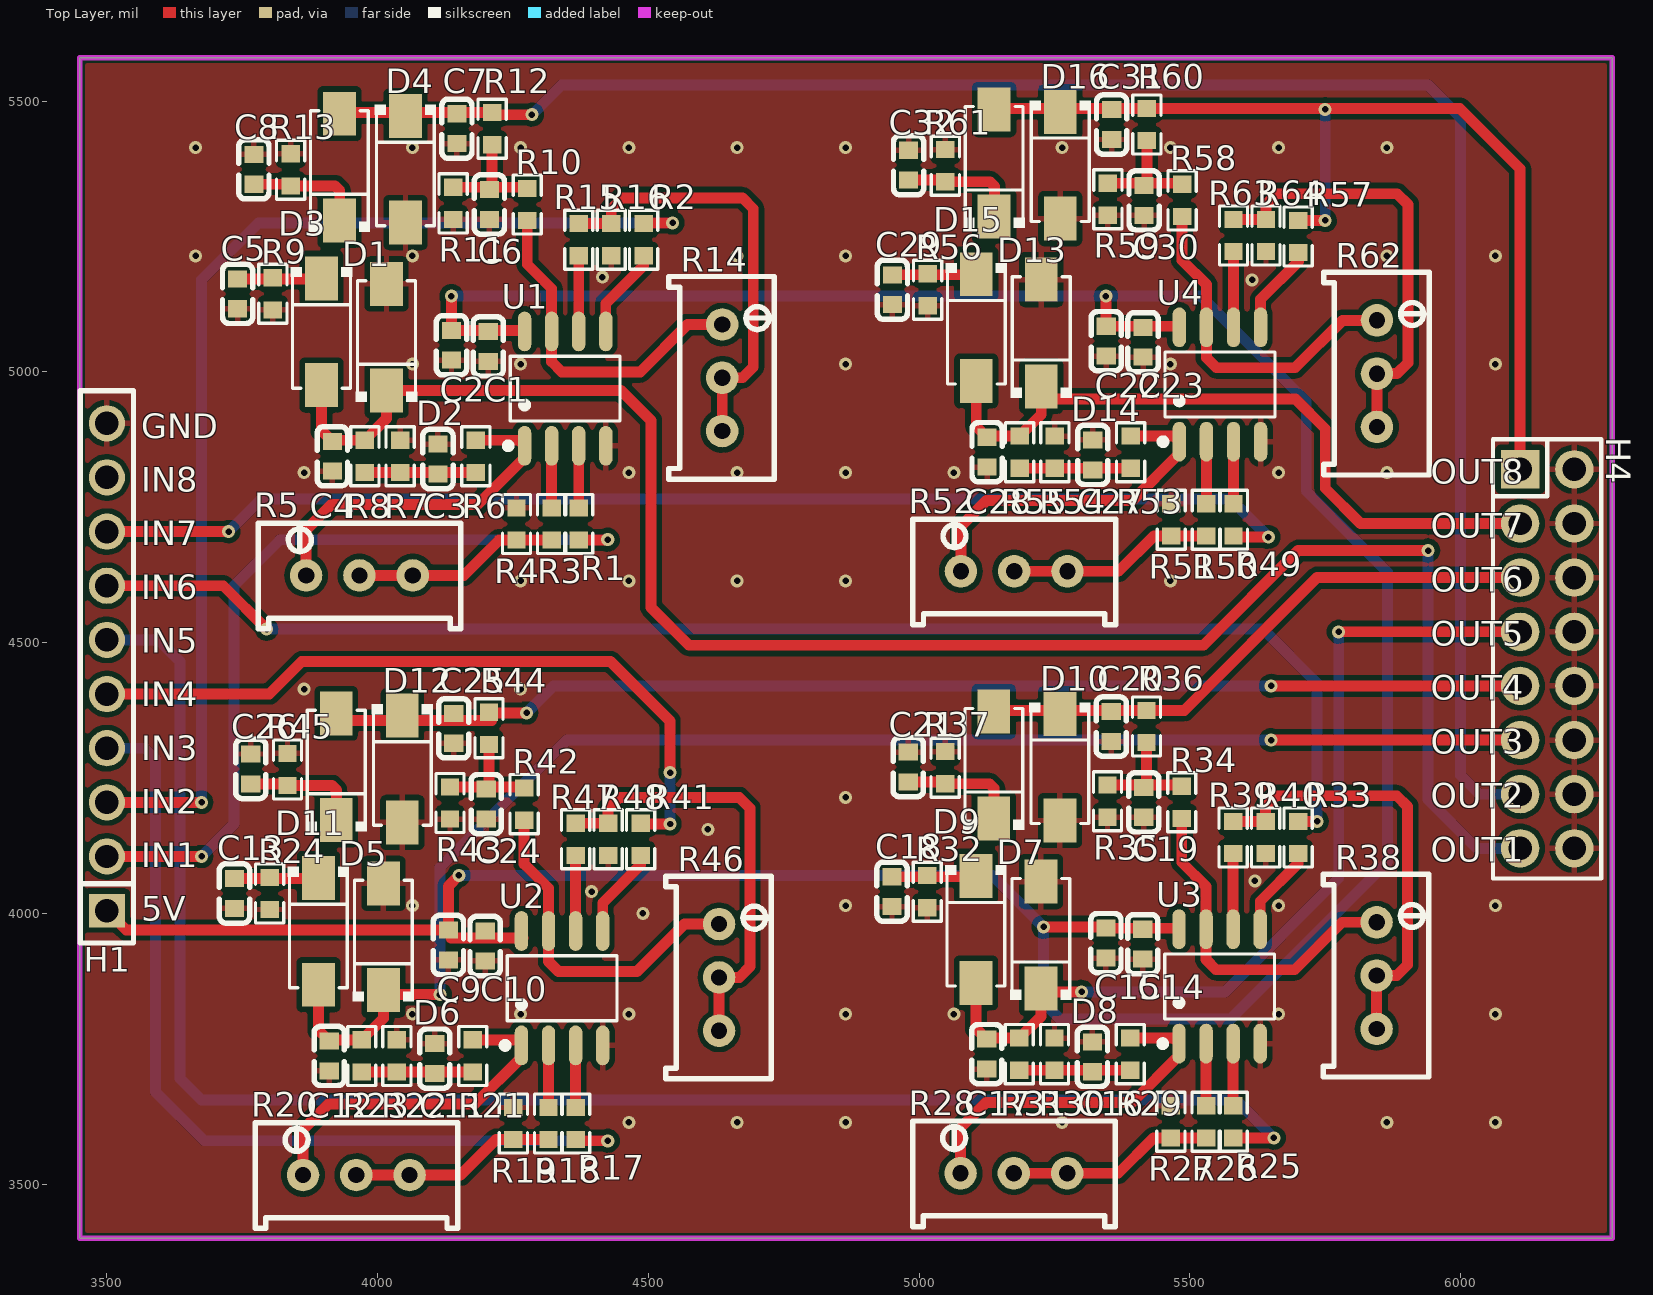
[diagram p0: Top Layer view]
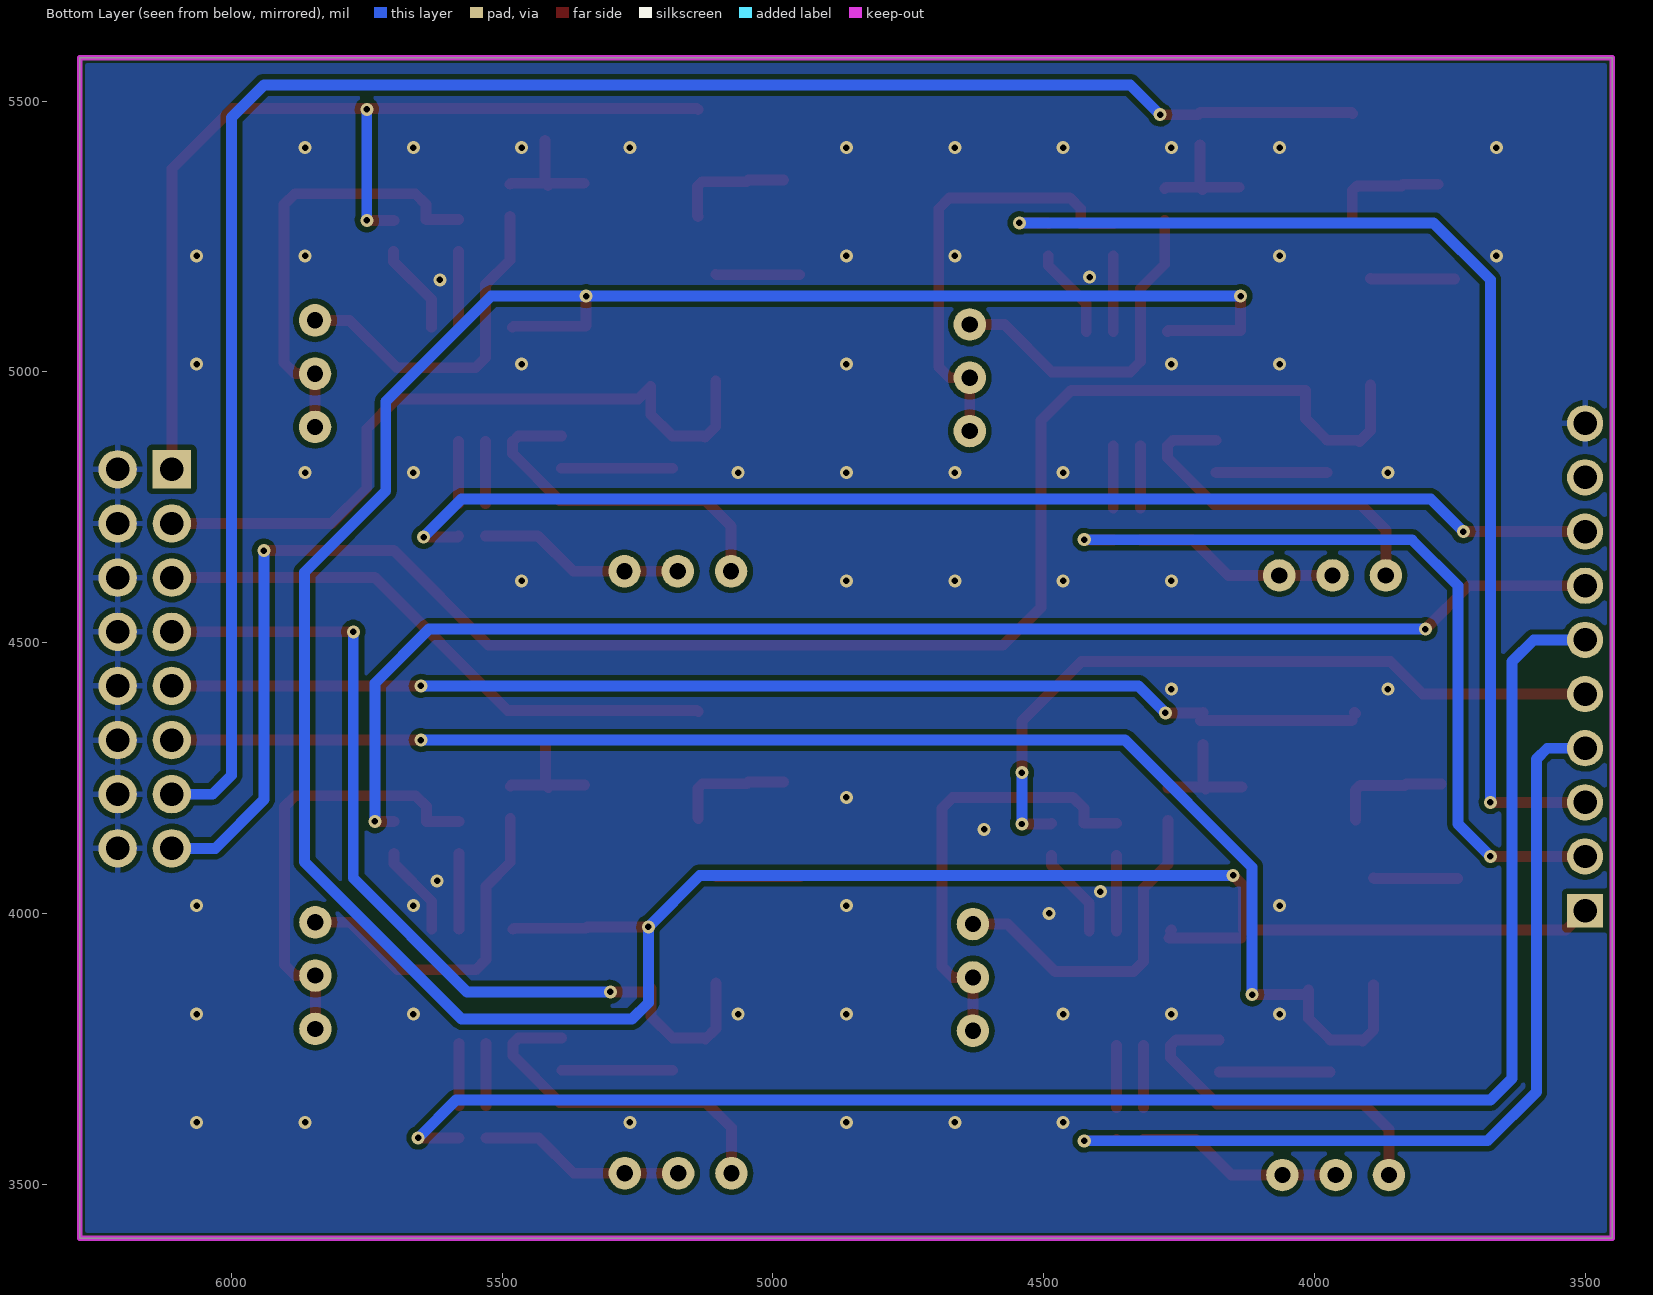
[diagram p1: Bottom Layer view, seen from below]
# Altium PCB MISC49941.pcbdoc
Units mil, origin at the board's own origin, x right, y up, seen from the top; angles counter-clockwise.
Board outline 2830 x 2180 mil, 2 copper layers (Top Layer, Bottom Layer), stack 62.206 mil thick; 118 components, 66 nets, 290 pads, 85 vias.

## Layer stack, top to bottom
Top Solder Mask Layer: solder mask 0.394, Dk 3.3
Top Layer: signal copper 1.379
Dielectric1: surface 59.449, FR4, Dk 4.5
Bottom Layer: signal copper 1.378
Bottom Solder Mask Layer: solder mask 0.394, Dk 3.3

## Board outline
3450,5580 3450,3400 6280,3400 6280,5580

## Design rules (kind name [scope] priority, off if disabled: settings)
BoardOutlineClearance copperThickness2oz_1 [All] p2 off: genericclearance=7.99 ignorepadtopadclearanceinfootprint=FALSE except(0: Arc-SplitContinuation Track-SplitContinuation SMDPad-SplitContinuation THPad-SplitContinuation Via-SplitContinuation Fill-SplitContinuation Region-SplitContinuation Poly-SplitContinuation Text-SplitContinuation Hole-SplitContinuation; 5.98: Arc-CutoutEdge SMDPad-CutoutEdge THPad-CutoutEdge Via-CutoutEdge Fill-CutoutEdge Region-CutoutEdge Text-CutoutEdge; 6.93: Hole-OutlineEdge Hole-CutoutEdge; 10: Poly-OutlineEdge Poly-CutoutEdge; 11.81: Arc-OutlineEdge Track-OutlineEdge SMDPad-OutlineEdge THPad-OutlineEdge Via-OutlineEdge Fill-OutlineEdge Region-OutlineEdge Text-OutlineEdge Track-CutoutEdge)
BoardOutlineClearance copperThickness1oz_1 [All] p4: genericclearance=4.02 ignorepadtopadclearanceinfootprint=FALSE except(0: Arc-SplitContinuation Track-SplitContinuation SMDPad-SplitContinuation THPad-SplitContinuation Via-SplitContinuation Fill-SplitContinuation Region-SplitContinuation Poly-SplitContinuation Text-SplitContinuation Hole-SplitContinuation; 6: SMDPad-CutoutEdge THPad-CutoutEdge Via-CutoutEdge Fill-CutoutEdge Region-CutoutEdge Text-CutoutEdge; 6.93: Hole-OutlineEdge Hole-CutoutEdge; 10: Poly-OutlineEdge Poly-CutoutEdge; 11.8: Arc-OutlineEdge Track-OutlineEdge SMDPad-OutlineEdge THPad-OutlineEdge Via-OutlineEdge Fill-OutlineEdge Region-OutlineEdge Text-OutlineEdge; 11.81: Arc-CutoutEdge Track-CutoutEdge)
Clearance copperThickness2oz [All] p1 off: gap=7.99 ignorepadtopadclearanceinfootprint=FALSE except(5.98: SMDPad-Track SMDPad-SMDPad THPad-Track SMDPad-THPad THPad-THPad Track-Via SMDPad-Via THPad-Via Via-Via Fill-Track Region-Track Fill-SMDPad Region-SMDPad Fill-THPad Region-THPad Fill-Via Region-Via Fill-Fill Fill-Region Region-Region Arc-Track Arc-SMDPad Arc-THPad Arc-Via Fill-Arc Region-Arc Arc-Arc Text-Track SMDPad-Text Text-THPad Text-Via Fill-Text Region-Text Arc-Text Text-Text; 6.93: Hole-Track Hole-SMDPad Hole-THPad Hole-Via Fill-Hole Region-Hole Hole-Arc Hole-Text; 10: Poly-Track Poly-SMDPad Poly-THPad Poly-Via Poly-Fill Poly-Region Poly-Poly Poly-Arc Poly-Text Poly-Hole)
Clearance copperThickness1oz [All] p3: gap=4.02 ignorepadtopadclearanceinfootprint=FALSE except(5.98: SMDPad-Track SMDPad-SMDPad THPad-Track SMDPad-THPad THPad-THPad Track-Via SMDPad-Via THPad-Via Via-Via Fill-Track Region-Track Fill-SMDPad Region-SMDPad Fill-THPad Region-THPad Fill-Via Region-Via Fill-Fill Fill-Region Region-Region; 6: Arc-Track Arc-SMDPad Arc-THPad Arc-Via Fill-Arc Region-Arc Arc-Arc Text-Track SMDPad-Text Text-THPad Text-Via Fill-Text Region-Text Arc-Text Text-Text; 6.93: Hole-Track Hole-SMDPad Hole-THPad Hole-Via Fill-Hole Region-Hole Hole-Arc Hole-Text; 10: Poly-Track Poly-SMDPad Poly-THPad Poly-Via Poly-Fill Poly-Region Poly-Poly Poly-Arc Poly-Text Poly-Hole)
Creepage creepage [All] p1: checkdistance=0 ignoreinternallayers=TRUE applytopolygonpour=TRUE
DiffPairsRouting differentialPair [All] p1: maxlimit=6 minlimit=6 mostfreqgap=6 toplayer_minwidth=5 toplayer_prefwidth=10 toplayer_maxwidth=100 toplayer_mingap=6 toplayer_prefgap=6 toplayer_maxgap=6 bottomlayer_minwidth=5 bottomlayer_prefwidth=10 bottomlayer_maxwidth=100 bottomlayer_mingap=6 bottomlayer_prefgap=6 bottomlayer_maxgap=6 maxuncoupledlength=10
HoleToHoleClearance otherClearance [All] p1: gap=11.81 allowstackedmicrovias=TRUE
Length netLength [All] p1: minlimit=0 maxlimit=0
MatchedLengths netLengthTolerance [All] p1: tolerance=1000
PasteMaskExpansion pasteMaskExpansion [All] p1: expansion=0
PlaneConnect innerPlane [All] p1: planeconnectstyle=Relief reliefexpansion=20 reliefentries=4 reliefconductorwidth=10 reliefairgap=10
PolygonConnect copperRegion [(InNet('GND'))] p1: connectstyle=Relief reliefconductorwidth=10 reliefentries=4 polygonreliefangle="90 Angle" airgapwidth=10 via.connectstyle=Relief via.reliefconductorwidth=10 via.reliefentries=4 via.polygonreliefangle="90 Angle" via.airgapwidth=10
RoutingVias viaSize [All] p1: holewidth=12.01 width=24.02 viastyle="Through Hole" minholewidth=11.81 minwidth=19.68 maxholewidth=248.03 maxwidth=393.7
SolderMaskExpansion solderMaskExpansion [IsVia] p1: expansion=-1000 istentingtop=TRUE
SolderMaskExpansion solderMaskExpansion [All] p2: expansion=2 istentingtop=FALSE
Width copperThickness2oz_2 [All] p1 off: maxlimit=100 minlimit=8 preferedwidth=10
Width copperThickness1oz_2 [All] p2: maxlimit=100 minlimit=5 preferedwidth=10

## Components (designator, comment, footprint, x,y, rotation, side; value= is the part's Value field where it differs from the comment)
C1 "100nF" C0603 4204.38,5047.12 r90 top
C2 "10uF" C0603 4136.4,5049.1 r90 top
C3 "10uF" C0603 4111.4,4839.1 r270 top
C4 "100nF" C0603 3916.4,4844.1 r90 top
C5 "100nF" C0603 3741.4,5144.1 r90 top
C6 "10uF" C0603 4206.4,5309.1 r90 top
C7 "100nF" C0603 4146.4,5449.1 r90 top
C8 "100nF" C0603 3771.4,5374.1 r270 top
C9 "100nF" C0603 4130.63,3941.71 r90 top
C10 "10uF" C0603 4198.61,3939.74 r90 top
C11 "10uF" C0603 4105.63,3731.71 r270 top
C12 "100nF" C0603 3910.63,3736.71 r90 top
C13 "100nF" C0603 3735.63,4036.71 r90 top
C14 "100nF" C0603 5412.98,3943.02 r90 top
C15 "10uF" C0603 5344.99,3945 r90 top
C16 "10uF" C0603 5319.99,3735 r270 top
C17 "100nF" C0603 5124.99,3740 r90 top
C18 "100nF" C0603 4949.99,4040 r90 top
C19 "10uF" C0603 5414.99,4205 r90 top
C20 "100nF" C0603 5354.99,4345 r90 top
C21 "100nF" C0603 4979.99,4270 r270 top
C22 "100nF" C0603 5345.63,5056.71 r90 top
C23 "10uF" C0603 5413.61,5054.74 r90 top
C24 "10uF" C0603 4200.63,4201.71 r90 top
C25 "100nF" C0603 4140.63,4341.71 r90 top
C26 "100nF" C0603 3765.63,4266.71 r270 top
C27 "10uF" C0603 5320.63,4846.71 r270 top
C28 "100nF" C0603 5125.63,4851.71 r90 top
C29 "100nF" C0603 4950.63,5151.71 r90 top
C30 "10uF" C0603 5415.63,5316.71 r90 top
C31 "100nF" C0603 5355.63,5456.71 r90 top
C32 "100nF" C0603 4980.63,5381.71 r270 top
D1 "SS54" SMA_L4.4-W2.8-LS5.4-R-RD 3896.4,5074.1 r270 top
D2 "SS54" SMA_L4.4-W2.8-LS5.4-R-RD 4016.4,5064.1 r90 top
D3 "SS54" SMA_L4.4-W2.8-LS5.4-R-RD 3929.38,5378.12 r90 top
D4 "SS54" SMA_L4.4-W2.8-LS5.4-R-RD 4051.4,5374.1 r270 top
D5 "SS54" SMA_L4.4-W2.8-LS5.4-R-RD 3890.63,3966.71 r270 top
D6 "SS54" SMA_L4.4-W2.8-LS5.4-R-RD 4010.63,3956.71 r90 top
D7 "SS54" SMA_L4.4-W2.8-LS5.4-R-RD 5104.99,3970 r270 top
D8 "SS54" SMA_L4.4-W2.8-LS5.4-R-RD 5224.99,3960 r90 top
D9 "SS54" SMA_L4.4-W2.8-LS5.4-R-RD 5137.98,4274.02 r90 top
D10 "SS54" SMA_L4.4-W2.8-LS5.4-R-RD 5259.99,4270 r270 top
D11 "SS54" SMA_L4.4-W2.8-LS5.4-R-RD 3923.61,4270.74 r90 top
D12 "SS54" SMA_L4.4-W2.8-LS5.4-R-RD 4045.63,4266.71 r270 top
D13 "SS54" SMA_L4.4-W2.8-LS5.4-R-RD 5105.63,5081.71 r270 top
D14 "SS54" SMA_L4.4-W2.8-LS5.4-R-RD 5225.63,5071.71 r90 top
D15 "SS54" SMA_L4.4-W2.8-LS5.4-R-RD 5138.61,5385.74 r90 top
D16 "SS54" SMA_L4.4-W2.8-LS5.4-R-RD 5260.63,5381.71 r270 top
H1 "" HDR-TH_10P-P2.54-V-F 3500,4455 r90 top
H4 "" HDR-TH_16P-P2.54-V-F-R2-C8-S2.54-1 6160,4470 r270 top
R1 "10K" R0603 4371.4,4719.1 r90 top
R2 "10K" R0603 4491.4,5244.1 r270 top
R3 "10K" R0603 4321.4,4719.1 r90 top
R4 "1K" R0603 4256.4,4719.1 r270 top
R5 "10kΩ" RES-ADJ-TH_3P-L10.0-W10.0-P2.50-L 3966.4,4624.1 r0 top
R6 "1K" R0603 4181.4,4844.1 r90 top
R7 "10K" R0603 4041.4,4844.1 r270 top
R8 "1K" R0603 3976.4,4844.1 r90 top
R9 "10K" R0603 3806.4,5144.1 r270 top
R10 "1K" R0603 4276.4,5309.1 r270 top
R11 "10K" R0603 4139.38,5311.18 r90 top
R12 "1K" R0603 4211.4,5449.1 r90 top
R13 "10K" R0603 3839.38,5373.12 r90 top
R14 "10kΩ" RES-ADJ-TH_3P-L10.0-W10.0-P2.50-L 4636.4,4989.1 r270 top
R15 "10K" R0603 4371.4,5244.1 r270 top
R16 "1K" R0603 4431.4,5244.1 r90 top
R17 "10K" R0603 4365.63,3611.71 r90 top
R18 "10K" R0603 4315.63,3611.71 r90 top
R19 "1K" R0603 4250.63,3611.71 r270 top
R20 "10kΩ" RES-ADJ-TH_3P-L10.0-W10.0-P2.50-L 3960.63,3516.71 r0 top
R21 "1K" R0603 4175.63,3736.71 r90 top
R22 "10K" R0603 4035.63,3736.71 r270 top
R23 "1K" R0603 3970.63,3736.71 r90 top
R24 "10K" R0603 3800.63,4036.71 r270 top
R25 "10K" R0603 5579.99,3615 r90 top
R26 "10K" R0603 5529.99,3615 r90 top
R27 "1K" R0603 5464.99,3615 r270 top
R28 "10kΩ" RES-ADJ-TH_3P-L10.0-W10.0-P2.50-L 5174.99,3520 r0 top
R29 "1K" R0603 5389.99,3740 r90 top
R30 "10K" R0603 5249.99,3740 r270 top
R31 "1K" R0603 5184.99,3740 r90 top
R32 "10K" R0603 5014.99,4040 r270 top
R33 "10K" R0603 5699.99,4140 r270 top
R34 "1K" R0603 5484.99,4205 r270 top
R35 "10K" R0603 5347.98,4207.08 r90 top
R36 "1K" R0603 5419.99,4345 r90 top
R37 "10K" R0603 5047.98,4269.02 r90 top
R38 "10kΩ" RES-ADJ-TH_3P-L10.0-W10.0-P2.50-L 5844.99,3885 r270 top
R39 "10K" R0603 5579.99,4140 r270 top
R40 "1K" R0603 5639.99,4140 r90 top
R41 "10K" R0603 4485.63,4136.71 r270 top
R42 "1K" R0603 4270.63,4201.71 r270 top
R43 "10K" R0603 4133.61,4203.8 r90 top
R44 "1K" R0603 4205.63,4341.71 r90 top
R45 "10K" R0603 3833.61,4265.74 r90 top
R46 "10kΩ" RES-ADJ-TH_3P-L10.0-W10.0-P2.50-L 4630.63,3881.71 r270 top
R47 "10K" R0603 4365.63,4136.71 r270 top
R48 "1K" R0603 4425.63,4136.71 r90 top
R49 "10K" R0603 5580.63,4726.71 r90 top
R50 "10K" R0603 5530.63,4726.71 r90 top
R51 "1K" R0603 5465.63,4726.71 r270 top
R52 "10kΩ" RES-ADJ-TH_3P-L10.0-W10.0-P2.50-L 5175.63,4631.71 r0 top
R53 "1K" R0603 5390.63,4851.71 r90 top
R54 "10K" R0603 5250.63,4851.71 r270 top
R55 "1K" R0603 5185.63,4851.71 r90 top
R56 "10K" R0603 5015.63,5151.71 r270 top
R57 "10K" R0603 5700,5250 r270 top
R58 "1K" R0603 5485.63,5316.71 r270 top
R59 "10K" R0603 5348.61,5318.8 r90 top
R60 "1K" R0603 5420.63,5456.71 r90 top
R61 "10K" R0603 5048.61,5380.74 r90 top
R62 "10kΩ" RES-ADJ-TH_3P-L10.0-W10.0-P2.50-L 5845.63,4996.71 r270 top
R63 "10K" R0603 5580.63,5251.71 r270 top
R64 "1K" R0603 5640.63,5251.71 r90 top
U1 "LM358DR-CN" SOIC-8_L4.9-W4.0-P1.27-LS6.0-BL 4346.4,4969.1 r0 top
U2 "LM358DR-CN" SOIC-8_L4.9-W4.0-P1.27-LS6.0-BL 4340.63,3861.71 r0 top
U3 "LM358DR-CN" SOIC-8_L4.9-W4.0-P1.27-LS6.0-BL 5554.99,3865 r0 top
U4 "LM358DR-CN" SOIC-8_L4.9-W4.0-P1.27-LS6.0-BL 5555.63,4976.71 r0 top

## Footprints (in the part's own frame and the unit in brackets; to place one, negate y for a bottom-side part, rotate by r counter-clockwise, add the part's x,y. Pads: shape width x height; smd on the part's side, far side on the other; paste and mask are expansions set on the pad)
C0603 [mm]
  rect 0.8x0.9 smd: 1(-0.7,0) 2(0.7,0)
  silkscreen extent -1.39,-0.71 1.39,0.71
HDR-TH_10P-P2.54-V-F [mm]
  rect 1.575x1.7 hole 1.1: 1(-11.43,0)
  round 1.7 hole 1.1: 2(-8.89,0) 3(-6.35,0) 4(-3.81,0) 5(-1.27,0) 6(1.27,0) 7(3.81,0) 8(6.35,0) 9(8.89,0) 10(11.43,0)
  silkscreen extent -12.95,-1.25 12.95,1.25
HDR-TH_16P-P2.54-V-F-R2-C8-S2.54-1 [mm]
  rect 1.8x1.8 hole 1.1: 1(-8.89,-1.27)
  round 1.8 hole 1.1: 2(-8.89,1.27) 3(-6.35,-1.27) 4(-6.35,1.27) 5(-3.81,-1.27) 6(-3.81,1.27) 7(-1.27,-1.27) 8(-1.27,1.27) 9(1.27,-1.27) 10(1.27,1.27) 11(3.81,-1.27) 12(3.81,1.27) 13(6.35,-1.27) 14(6.35,1.27) 15(8.89,-1.27) 16(8.89,1.27)
  silkscreen extent -10.3,-2.54 10.3,2.54
R0603 [mil]
  rect 31.75x34.02 smd paste-3937.01 mask+2: 1(-29.66,0) 2(29.66,0)
  silkscreen extent -55,-26 55,26
RES-ADJ-TH_3P-L10.0-W10.0-P2.50-L [mil]
  round 60 hole 30: 1(-98.43,0) 2(0,0) 3(98.42,0)
  silkscreen extent -187,-98 187,96
SMA_L4.4-W2.8-LS5.4-R-RD [mil]
  rect 81.2x60.59 smd: 1(98.57,0) 2(-98.57,0)
  silkscreen extent -119,-56 104,56
SOIC-8_L4.9-W4.0-P1.27-LS6.0-BL [mm]
  oval 0.63x1.865 smd: 1(-1.905,-2.682) 2(-0.635,-2.682) 3(0.635,-2.682) 4(1.905,-2.682) 5(1.905,2.682) 6(0.635,2.682) 7(-0.635,2.682) 8(-1.905,2.682)
  silkscreen extent -2.82,-2.83 2.58,1.52

## Via types
v1: diameter 24.02, hole 12, Top Layer to Bottom Layer, 85 vias

## Nets (pads, with @x,y where several pads share a name; then routed paths per layer and width w, separated by ;. In a path a pad name is that pad's centre, name@x,y a point inside that pad or via, vN(x,y) a via of type N, cw(c..) or ccw(c..) an arc to the next point about the centre after c; other vN are vias at no path point)
$1N5: C8.2 D3.2 R13.1 | length 219.1
  Top Layer w20: C8.2 3836.3,5346.54 R13.1 3921.54,5343.46 3930,5335 3930,5280.16 D3.2
$1N8: C5.2 D1.2 R9.1 | length 155.4
  Top Layer w20: C5.2 3895.39,5171.66 D1.2
$1N9: R14.2 R14.3 R15.1 R16.2 | length 822.6
  Top Layer w20: R15.1 R16.2 4431.4,5301.4 4451.4,5321.4 4673.6,5321.4 4693.6,5301.4 4693.6,5009.09 4673.6,4989.09 R14.2 R14.3
$1N10: R15.2 U1.6 | length 139.7
  Top Layer w20: U1.6 R15.2
$1N11: R10.2 R14.1 U1.7 | length 638.4
  Top Layer w20: R10.2 4276.4,5198.6 4321.4,5153.6 U1.7 4321.4,5018.6 4340,5000 4485,5000 4572.52,5087.52 R14.1
$1N15: C6.2 R10.1 R11.2 R12.1 | length 222.7
  Top Layer w20: R11.2 C6.2@4210.59,5340.84 ; C6.2 C6.2@4210.59,5340.84 ; R12.1 4211.4,5341.66 C6.2@4210.59,5340.84 ; R10.1 4274.32,5340.84 C6.2@4210.59,5340.84
$1N18: C3.2 R6.1 R7.2 R8.1 | length 205
  Top Layer w20: R8.1 R7.2 R6.1
$1N21: R5.1 R6.2 U1.1 | length 658.9
  Top Layer w20: R5.1 3867.98,4707.98 3915,4755 4185,4755 4271.4,4841.4 U1.1 4261.13,4873.76 R6.2
$1N22: R3.1 R4.2 R5.2 R5.3 | length 382.1
  Top Layer w20: R5.2 R5.3 4159.1,4624.1 4224.44,4689.44 R4.2 R3.1
$1N23: R3.2 U1.2 | length 114.7
  Top Layer w20: R3.2 U1.2
$1N26: R2.2 U1.5 | length 168.7
  Top Layer w20: U1.5 4421.4,5126.4 4491.4,5196.4 R2.2
$1N27: R1.2 U1.3 | length 114.7
  Top Layer w20: R1.2 U1.3
$1N31: C26.2 D11.2 R45.1 | length 219.1
  Top Layer w20: C26.2 3830.53,4239.15 R45.1 3915.77,4236.08 3924.22,4227.62 3924.22,4172.78 D11.2
$1N33: R46.2 R46.3 R47.1 R48.2 | length 822.6
  Top Layer w20: R47.1 R48.2 4425.63,4194.02 4445.63,4214.02 4667.82,4214.02 4687.82,4194.02 4687.82,3901.71 4667.82,3881.71 R46.2 R46.3
$1N34: R47.2 U2.6 | length 139.7
  Top Layer w20: U2.6 R47.2
$1N35: R42.2 R46.1 U2.7 | length 638.4
  Top Layer w20: R42.2 4270.63,4091.22 4315.63,4046.21 U2.7 4315.63,3911.21 4334.22,3892.62 4479.22,3892.62 4566.75,3980.14 R46.1
$1N39: C24.2 R42.1 R43.2 R44.1 | length 222.7
  Top Layer w20: R43.2 C24.2@4204.81,4233.46 ; C24.2 C24.2@4204.81,4233.46 ; R44.1 4205.63,4234.27 C24.2@4204.81,4233.46 ; R42.1 4268.54,4233.46 C24.2@4204.81,4233.46
$1N40: R41.2 U2.5 | length 168.7
  Top Layer w20: U2.5 4415.63,4019.02 4485.63,4089.02 R41.2
$1N43: C13.2 D5.2 R24.1 | length 155.4
  Top Layer w20: C13.2 3889.62,4064.27 D5.2
$1N47: C11.2 R21.1 R22.2 R23.1 | length 205
  Top Layer w20: R23.1 R22.2 R21.1
$1N49: R20.1 R21.2 U2.1 | length 658.9
  Top Layer w20: R20.1 3862.2,3600.59 3909.22,3647.62 4179.22,3647.62 4265.63,3734.02 U2.1 4255.36,3766.37 R21.2
$1N50: R18.1 R19.2 R20.2 R20.3 | length 382.1
  Top Layer w20: R20.2 R20.3 4153.32,3516.71 4218.66,3582.05 R19.2 R18.1
$1N51: R18.2 U2.2 | length 114.7
  Top Layer w20: R18.2 U2.2
$1N54: R17.2 U2.3 | length 114.7
  Top Layer w20: R17.2 U2.3
$1N58: C21.2 D9.2 R37.1 | length 219.1
  Top Layer w20: C21.2 5044.9,4242.44 R37.1 5130.14,4239.36 5138.59,4230.9 5138.59,4176.07 D9.2
$1N60: R38.2 R38.3 R39.1 R40.2 | length 822.6
  Top Layer w20: R39.1 R40.2 5639.99,4197.3 5659.99,4217.3 5882.19,4217.3 5902.19,4197.3 5902.19,3904.99 5882.19,3884.99 R38.2 R38.3
$1N61: R39.2 U3.6 | length 139.7
  Top Layer w20: U3.6 R39.2
$1N62: R34.2 R38.1 U3.7 | length 638.4
  Top Layer w20: R34.2 5484.99,4094.5 5530,4049.5 U3.7 5530,3914.5 5548.59,3895.9 5693.59,3895.9 5781.12,3983.43 R38.1
$1N66: C19.2 R34.1 R35.2 R36.1 | length 222.7
  Top Layer w20: R35.2 C19.2@5419.18,4236.74 ; C19.2 C19.2@5419.18,4236.74 ; R36.1 5419.99,4237.56 C19.2@5419.18,4236.74 ; R34.1 5482.91,4236.74 C19.2@5419.18,4236.74
$1N67: R33.2 U3.5 | length 168.7
  Top Layer w20: U3.5 5630,4022.31 5699.99,4092.3 R33.2
$1N70: C18.2 D7.2 R32.1 | length 155.4
  Top Layer w20: C18.2 5103.98,4067.56 D7.2
$1N74: C16.2 R29.1 R30.2 R31.1 | length 205
  Top Layer w20: R31.1 R30.2 R29.1
$1N76: R28.1 R29.2 U3.1 | length 658.9
  Top Layer w20: R28.1 5076.57,3603.88 5123.59,3650.9 5393.59,3650.9 5480,3737.31 U3.1 5469.73,3769.66 R29.2
$1N77: R26.1 R27.2 R28.2 R28.3 | length 382.1
  Top Layer w20: R28.2 R28.3 5367.69,3520 5433.03,3585.34 R27.2 R26.1
$1N78: R26.2 U3.2 | length 114.7
  Top Layer w20: R26.2 U3.2
$1N81: R25.2 U3.3 | length 114.7
  Top Layer w20: R25.2 U3.3
$1N85: C32.2 D15.2 R61.1 | length 219.1
  Top Layer w20: C32.2 5045.53,5354.15 R61.1 5130.77,5351.08 5139.22,5342.62 5139.22,5287.78 D15.2
$1N87: R62.2 R62.3 R63.1 R64.2 | length 822.6
  Top Layer w20: R63.1 R64.2 5640.63,5309.02 5660.63,5329.02 5882.82,5329.02 5902.82,5309.02 5902.82,5016.71 5882.82,4996.71 R62.2 R62.3
$1N88: R63.2 U4.6 | length 139.7
  Top Layer w20: U4.6 R63.2
$1N89: R58.2 R62.1 U4.7 | length 638.4
  Top Layer w20: R58.2 5485.63,5206.22 5530.63,5161.21 U4.7 5530.63,5026.21 5549.22,5007.62 5694.22,5007.62 5781.75,5095.14 R62.1
$1N93: C30.2 R58.1 R59.2 R60.1 | length 222.7
  Top Layer w20: R59.2 C30.2@5419.81,5348.46 ; C30.2 C30.2@5419.81,5348.46 ; R60.1 5420.63,5349.27 C30.2@5419.81,5348.46 ; R58.1 5483.54,5348.46 C30.2@5419.81,5348.46
$1N94: R57.2 U4.5 | length 168.7
  Top Layer w20: U4.5 5630.63,5134.02 5700.63,5204.02 R57.2@5700.63,5222.05
$1N97: C29.2 D13.2 R56.1 | length 155.4
  Top Layer w20: C29.2 5104.62,5179.27 D13.2
$1N101: C27.2 R53.1 R54.2 R55.1 | length 205
  Top Layer w20: R55.1 R54.2 R53.1
$1N103: R52.1 R53.2 U4.1 | length 658.9
  Top Layer w20: R52.1 5077.2,4715.59 5124.22,4762.62 5394.22,4762.62 5480.63,4849.02 U4.1 5470.36,4881.37 R53.2
$1N104: R50.1 R51.2 R52.2 R52.3 | length 382.1
  Top Layer w20: R52.2 R52.3 5368.32,4631.71 5433.66,4697.05 R51.2 R50.1
$1N106: R50.2 U4.2 | length 114.7
  Top Layer w20: R50.2 U4.2
$1N109: R49.2 U4.3 | length 114.7
  Top Layer w20: R49.2 U4.3
+5V: C1.2 C2.2 C9.2 C10.2 C14.2 C15.2 C22.2 C23.2 H1.1 U1.8 U2.8 U3.8 U4.8 | length 6131.1
  Top Layer w20: H1.1 3535.73,3969.27 C9.2 4130.63,4050.63 v1(4150,4070) ; C9.2@4135.63,3954.27 U2.8@4268.68,3954.27 ; v1(4136.4,5140) C2.2 4269.45,5076.66 U1.8 ; U2.8@4263.68,3969.27 U2.8 ; v1(5230,3975) 5342.56,3975 C15.2 5478.05,3972.56 U3.8 ; v1(5345,5140) 5345,5084.9 C22.2 5478.68,5084.27 U4.8
  Bottom Layer w20: v1(4136.4,5140) v1(5345,5140) 5520,5140 5715,4945 5715,4780 5865,4630 5865,4095 5575,3805 5260,3805 5230,3835 v1(5230,3975) 5135,4070 v1(4150,4070)
GND: C1.1 C2.1 C3.1 C4.1 C5.1 C6.1 C7.1 C8.1 C9.1 C10.1 C11.1 C12.1 C13.1 C14.1 C15.1 C16.1 C17.1 C18.1 C19.1 C20.1 C21.1 C22.1 C23.1 C24.1 C25.1 C26.1 C27.1 C28.1 C29.1 C30.1 C31.1 C32.1 D2.1 D4.1 D6.1 D8.1 D10.1 D12.1 D14.1 D16.1 H1.10 H4.2 H4.4 H4.6 H4.8 H4.10 H4.12 H4.14 H4.16 R4.1 R7.1 R9.2 R11.1 R13.2 R16.1 R19.1 R22.1 R24.2 R27.1 R30.1 R32.2 R35.1 R37.2 R40.1 R43.1 R45.2 R48.1 R51.1 R54.1 R56.2 R59.1 R61.2 R64.1 U1.4 U2.4 U3.4 U4.4
  other v1: 4464.1,3614.1 4664.1,3614.1 4864.1,3614.1 5264.1,3614.1 5864.1,3614.1 6064.1,3614.1 4064.1,3814.1 4264.1,3814.1 4464.1,3814.1 4864.1,3814.1 5064.1,3814.1 5664.1,3814.1 6064.1,3814.1 4490,4000 4064.1,4014.1 4864.1,4014.1 5664.1,4014.1 6064.1,4014.1 4395,4040 5620,4060 4610,4155 4864.1,4214.1 3864.1,4414.1 4264.1,4414.1 4264.1,4614.1 4464.1,4614.1 4664.1,4614.1 4864.1,4614.1 5464.1,4614.1 3864.1,4814.1 4464.1,4814.1 4664.1,4814.1 4864.1,4814.1 5064.1,4814.1 5664.1,4814.1 5864.1,4814.1 4064.1,5014.1 4264.1,5014.1 4864.1,5014.1 5464.1,5014.1 6064.1,5014.1 5615,5170 4415,5175 3664.1,5214.1 4064.1,5214.1 4664.1,5214.1 4864.1,5214.1 5864.1,5214.1 6064.1,5214.1 3664.1,5414.1 4064.1,5414.1 4264.1,5414.1 4464.1,5414.1 4664.1,5414.1 4864.1,5414.1 5264.1,5414.1 5464.1,5414.1 5664.1,5414.1 5864.1,5414.1
IN1: H1.2 R1.1 | length 1478.9
  Top Layer w20: H1.2 v1(3675,4105) ; R1.1 4424.44,4689.44 v1(4425,4690)
  Bottom Layer w20: v1(3675,4105) 3735,4165 3735,4605 3820,4690 v1(4425,4690)
IN2: H1.3 R2.1 | length 2107.6
  Top Layer w20: H1.3 v1(3675,4205) ; R2.1 4492.64,5275 v1(4545,5275)
  Bottom Layer w20: v1(3675,4205) 3675,5170 3780,5275 v1(4545,5275)
IN3: H1.4 R17.1 | length 1645.8
  Top Layer w20: R17.1 4367.68,3580 v1(4425,3580)
  Bottom Layer w20: H1.4 3570,4305 3590,4285 3590,3670 3680,3580 v1(4425,3580)
IN4: H1.5 R41.1 | length 1355.4
  Top Layer w20: H1.5 3800,4405 3860,4465 4430,4465 4540,4355 v1(4540,4260) ; R41.1 4487,4165 v1(4540,4165)
  Bottom Layer w20: v1(4540,4165) v1(4540,4260)
IN5: H1.6 R25.1 | length 3062
  Top Layer w20: R25.1 v1(5655,3585.34)
  Bottom Layer w20: H1.6 3595,4505 3635,4465 3635,3695 3675,3655 5585.34,3655 v1(5655,3585.34)
IN6: H1.7 R33.1 | length 2599.7
  Top Layer w20: H1.7 3715,4605 v1(3795,4525) ; R33.1 5734.66,4169.66 v1(5735,4170)
  Bottom Layer w20: v1(3795,4525) 5635,4525 5735,4425 v1(5735,4170)
IN7: H1.8 R49.1 | length 2264.1
  Top Layer w20: H1.8 v1(3725,4705) ; R49.1 5582.68,4695 v1(5645,4695)
  Bottom Layer w20: v1(3725,4705) 3785,4765 5575,4765 v1(5645,4695)
IN8: H1.9
OUT1: C4.2 D1.1 D2.2 H4.15 R8.2 | length 3341.7
  Top Layer w20: D1.1 3896.4,4891.66 C4.2 3918.5,4873.76 R8.2 4016.4,4913.76 D2.2 4449.47,4965.53 4505,4910 4505,4565 4575,4495 5525,4495 5700,4670 v1(5940,4670)
  Bottom Layer w20: v1(5940,4670) 5940,4210 6030,4120 H4.15
OUT2: C7.2 D3.1 D4.2 H4.13 R12.2 | length 3460.2
  Top Layer w20: D3.1 3931.45,5478.76 R12.2 4215.16,5475 v1(4285,5475)
  Bottom Layer w20: v1(4285,5475) 4340,5530 5940,5530 6000,5470 6000,4255 6035,4220 H4.13
OUT3: C12.2 D5.1 D6.2 H4.11 R23.2 | length 2716.5
  Top Layer w20: D5.1 3890.63,3784.27 C12.2 3912.73,3766.37 R23.2 4010.63,3806.37 D6.2 4018.77,3850 v1(4115,3850) ; v1(5650,4320) H4.11
  Bottom Layer w20: v1(4115,3850) 4115,4085 4350,4320 v1(5650,4320)
OUT4: C25.2 D11.1 D12.2 H4.9 R44.2 | length 2208.5
  Top Layer w20: D11.1 D11.1@3925.68,4371.37 ; D11.1@3930.68,4356.37 R44.2@4210.63,4356.37 ; R44.2 4207,4370 v1(4275,4370) ; v1(5650,4420) H4.9
  Bottom Layer w20: v1(4275,4370) 4325,4420 v1(5650,4420)
OUT5: C17.2 D7.1 D8.2 H4.7 R31.2 | length 1711
  Top Layer w20: D7.1 5104.99,3787.56 C17.2 5127.1,3769.66 R31.2 5224.99,3809.66 D8.2 5231.43,3855 v1(5300,3855) ; v1(5775,4520) H4.7
  Bottom Layer w20: v1(5300,3855) 5565,3855 5775,4065 v1(5775,4520)
OUT6: C20.2 D9.1 D10.2 H4.5 R36.2 | length 1074.5
  Top Layer w20: D9.1 5140.05,4374.66 R36.2 5489.66,4374.66 5735,4620 H4.5
OUT7: C28.2 D13.1 D14.2 H4.3 R55.2 | length 1335
  Top Layer w20: D13.1 5105.63,4899.27 C28.2 5127.73,4881.37 R55.2 5225.63,4921.37 D14.2 5248.77,4950 5695,4950 5750,4895 5750,4785 5815,4720 H4.3
OUT8: C31.2 D15.1 D16.2 H4.1 R57.1 R60.2 | length 1828.7
  Top Layer w20: D15.1 5140.68,5486.37 R60.2 5998.63,5486.37 6110,5375 H4.1 ; R57.1 v1(5750,5279.66)
  Bottom Layer w20: v1(5750,5279.66) v1(5750,5485)

## Polygon pours and split planes (outlines as drawn)
GND on Top Layer (solid, remove dead copper, pour order 0): 3150,5815 3150,3000 6690,3000 6690,5815
GND on Bottom Layer (solid, remove dead copper, pour order 2): 3000,5745 3000,3195 6685,3195 6685,5745

## Keep-outs
Board Outline Layer:
  the board outline again, w10

## Silkscreen, mask and mechanical layers (free items; w line width, h text height)
Top Silkscreen Layer:
  text "GND" at 3563.6,4877.5 h45
  text "OUT8" at 5945,4793 h45
  text "IN8" at 3563.6,4778.43 h45
  text "OUT7" at 5945,4693.29 h45
  text "IN7" at 3563.6,4679.36 h45
  text "OUT6" at 5945,4593.57 h45
  text "IN6" at 3563.6,4580.3 h45
  text "OUT5" at 5945,4493.86 h45
  text "IN5" at 3563.6,4481.23 h45
  text "OUT4" at 5945,4394.14 h45
  text "IN4" at 3563.6,4382.16 h45
  text "OUT3" at 5945,4294.43 h45
  text "IN3" at 3563.6,4283.09 h45
  text "OUT2" at 5945,4194.71 h45
  text "IN2" at 3563.6,4184.03 h45
  text "OUT1" at 5945,4095 h45
  text "IN1" at 3563.6,4084.96 h45
  text "5V" at 3563.6,3985.89 h45